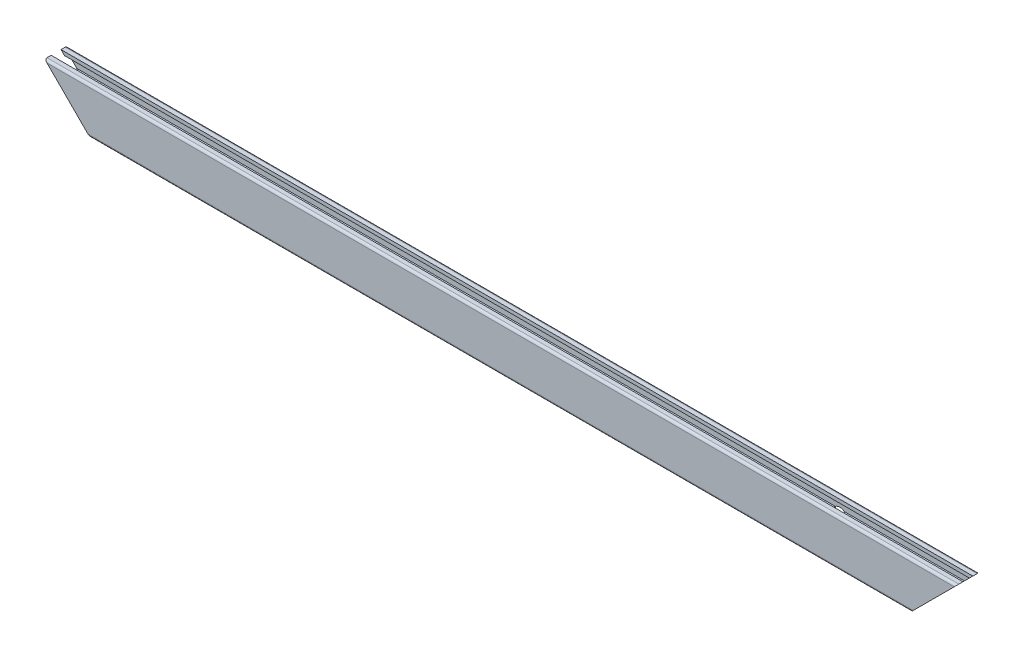
SolidWorks part; units mm, degrees
ref_plane "前视" through (0, 0, 0) normal (0, 0, 1) x (1, 0, 0)
ref_plane "上视" through (0, 0, 0) normal (0, 1, 0) x (1, 0, 0)
ref_plane "右视" through (0, 0, 0) normal (1, 0, 0) x (0, 0, -1)
sketch3d "3D草图1"
  line L0 (-300, 0, 0) -> (300, 0, 0)
  dimension "D1" = 600
other "结构构件1"
ref_plane "基准面1" through (-300, 0, 0) normal (1, 0, 0) x (0, 0, -1)
sketch "Sketch12" plane through (-300, 0, 0) normal (1, 0, 0) x (0, 0, -1)
  line L1 (0, 16.311) -> (0, -16.311) construction
  line L2 (0, 0) -> (9.513, 0) construction
  line L3 (-6, -15) -> (-3.25, -15)
  line L4 (-7.5, -13.5) -> (-7.5, 13.5)
  line L5 (-6, 15) -> (-3.25, 15)
  line L6 (7.5, -13.5) -> (7.5, 13.5)
  line L17 (3.25, 15) -> (6, 15)
  line L20 (-5.7, 12.7) -> (-5.7, 7)
  line L21 (-3.25, 12.7) -> (-5.7, 12.7)
  line L24 (5.7, 12.7) -> (5.7, 7)
  line L25 (3.25, 12.7) -> (5.7, 12.7)
  line L26 (-3.25, 15) -> (-3.25, 12.7)
  line L27 (3.25, 15) -> (3.25, 12.7)
  line L40 (5.7, -12.7) -> (5.7, -7)
  line L41 (3.25, -12.7) -> (5.7, -12.7)
  line L44 (-5.7, -12.7) -> (-5.7, -7)
  line L45 (-3.25, -12.7) -> (-5.7, -12.7)
  line L47 (3.25, -15) -> (3.25, -12.7)
  line L48 (-3.25, -15) -> (-3.25, -12.7)
  line L49 (3.25, -15) -> (6, -15)
  arc A0 (-6, -15) -> (-7.5, -13.5) centre (-6, -13.5) cw
  arc A1 (6, -15) -> (7.5, -13.5) centre (6, -13.5) ccw
  arc A2 (6, 15) -> (7.5, 13.5) centre (6, 13.5) cw
  arc A3 (-7.5, 13.5) -> (-6, 15) centre (-6, 13.5) cw
  circle A4 centre (0, 0) radius 2.5
  arc A5 (-5.7, 7) -> (5.7, 7) centre (0, 12.248) ccw
  arc A6 (-5.7, -7) -> (5.7, -7) centre (0, -12.248) cw
  point P4 (0, 0)
  point P21 (0, 0)
  point P44 (-7.5, 15)
  point P45 (7.5, 15)
  point P46 (7.5, -15)
  point P47 (-7.5, -15)
  point P48 (0, -15)
  point P49 (0, 15)
  dimension "D1" = 30
  dimension "D2" = 15
  dimension "D3" = 1.5
  dimension "D4" = 5
  dimension "D5" = 6.5
  dimension "D6" = 10.5
  dimension "D7" = 8
  dimension "D8" = 11.4
  dimension "D9" = 2.3
sketch "草图4" plane through (0, 0, 7.5) normal (0, 0, 1) x (1, 0, 0)
  line L0 (-300, 15) -> (-270, -15)
  line L2 (0, 0) -> (0, -85.0329) construction
  line L3 (-270, -15) -> (-300, -15)
  line L4 (-300, -15) -> (-300, 15)
  line L5 (300, -15) -> (300, 15)
  line L6 (270, -15) -> (300, -15)
  line L7 (300, 15) -> (270, -15)
  line L8 (300, 15) -> (-300, 15) construction
  line L9 (300, -15) -> (-300, -15) construction
  line L10 (-300, 13.5) -> (-300, -13.5) construction
extrude "切除-拉伸1" cut sketch "草图4" against normal through all
sketch "草图7" plane through (0, 0, -7.5) normal (0, 0, 1) x (1, 0, 0)
  line L0 (300, 15) -> (-300, 15) construction
  circle A0 centre (210, 3) radius 5
  dimension "D1" = 10
  dimension "D2" = 90
  dimension "D3" = 12
extrude "切除-拉伸2" cut sketch "草图7" along normal blind 4.999
